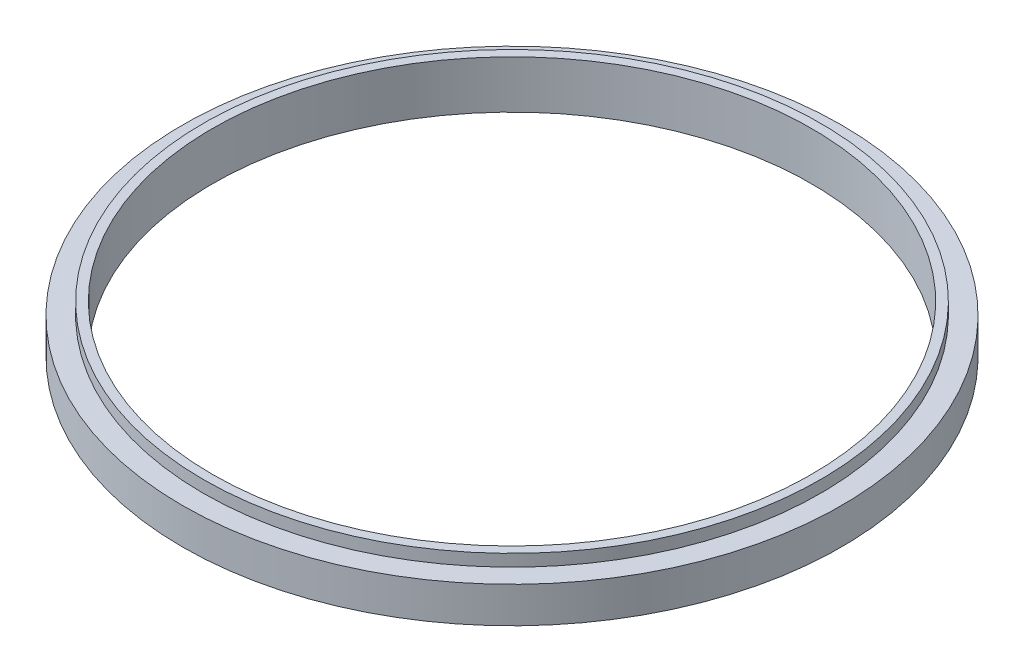
SolidWorks part; units mm, degrees
ref_plane "Front Plane" through (0, 0, 0) normal (0, 0, 1) x (1, 0, 0)
ref_plane "Top Plane" through (0, 0, 0) normal (0, 1, 0) x (1, 0, 0)
ref_plane "Right Plane" through (0, 0, 0) normal (1, 0, 0) x (0, 0, -1)
sketch "Sketch1" plane through (0, 0, 0) normal (0, 1, 0) x (1, 0, 0)
  circle A0 centre (0, 0) radius 55
  circle A1 centre (0, 0) radius 50
  dimension "D1" = 100
  dimension "D2" = 110
extrude "Boss-Extrude1" add sketch "Sketch1" along normal blind 6
sketch "Sketch2" plane through (0, 6, 0) normal (0, 1, 0) x (1, 0, 0)
  circle A0 centre (0, 0) radius 50
  circle A1 centre (0, 0) radius 51.5
  dimension "D1" = 100
  dimension "D2" = 103
extrude "Boss-Extrude2" add sketch "Sketch2" along normal blind 2
